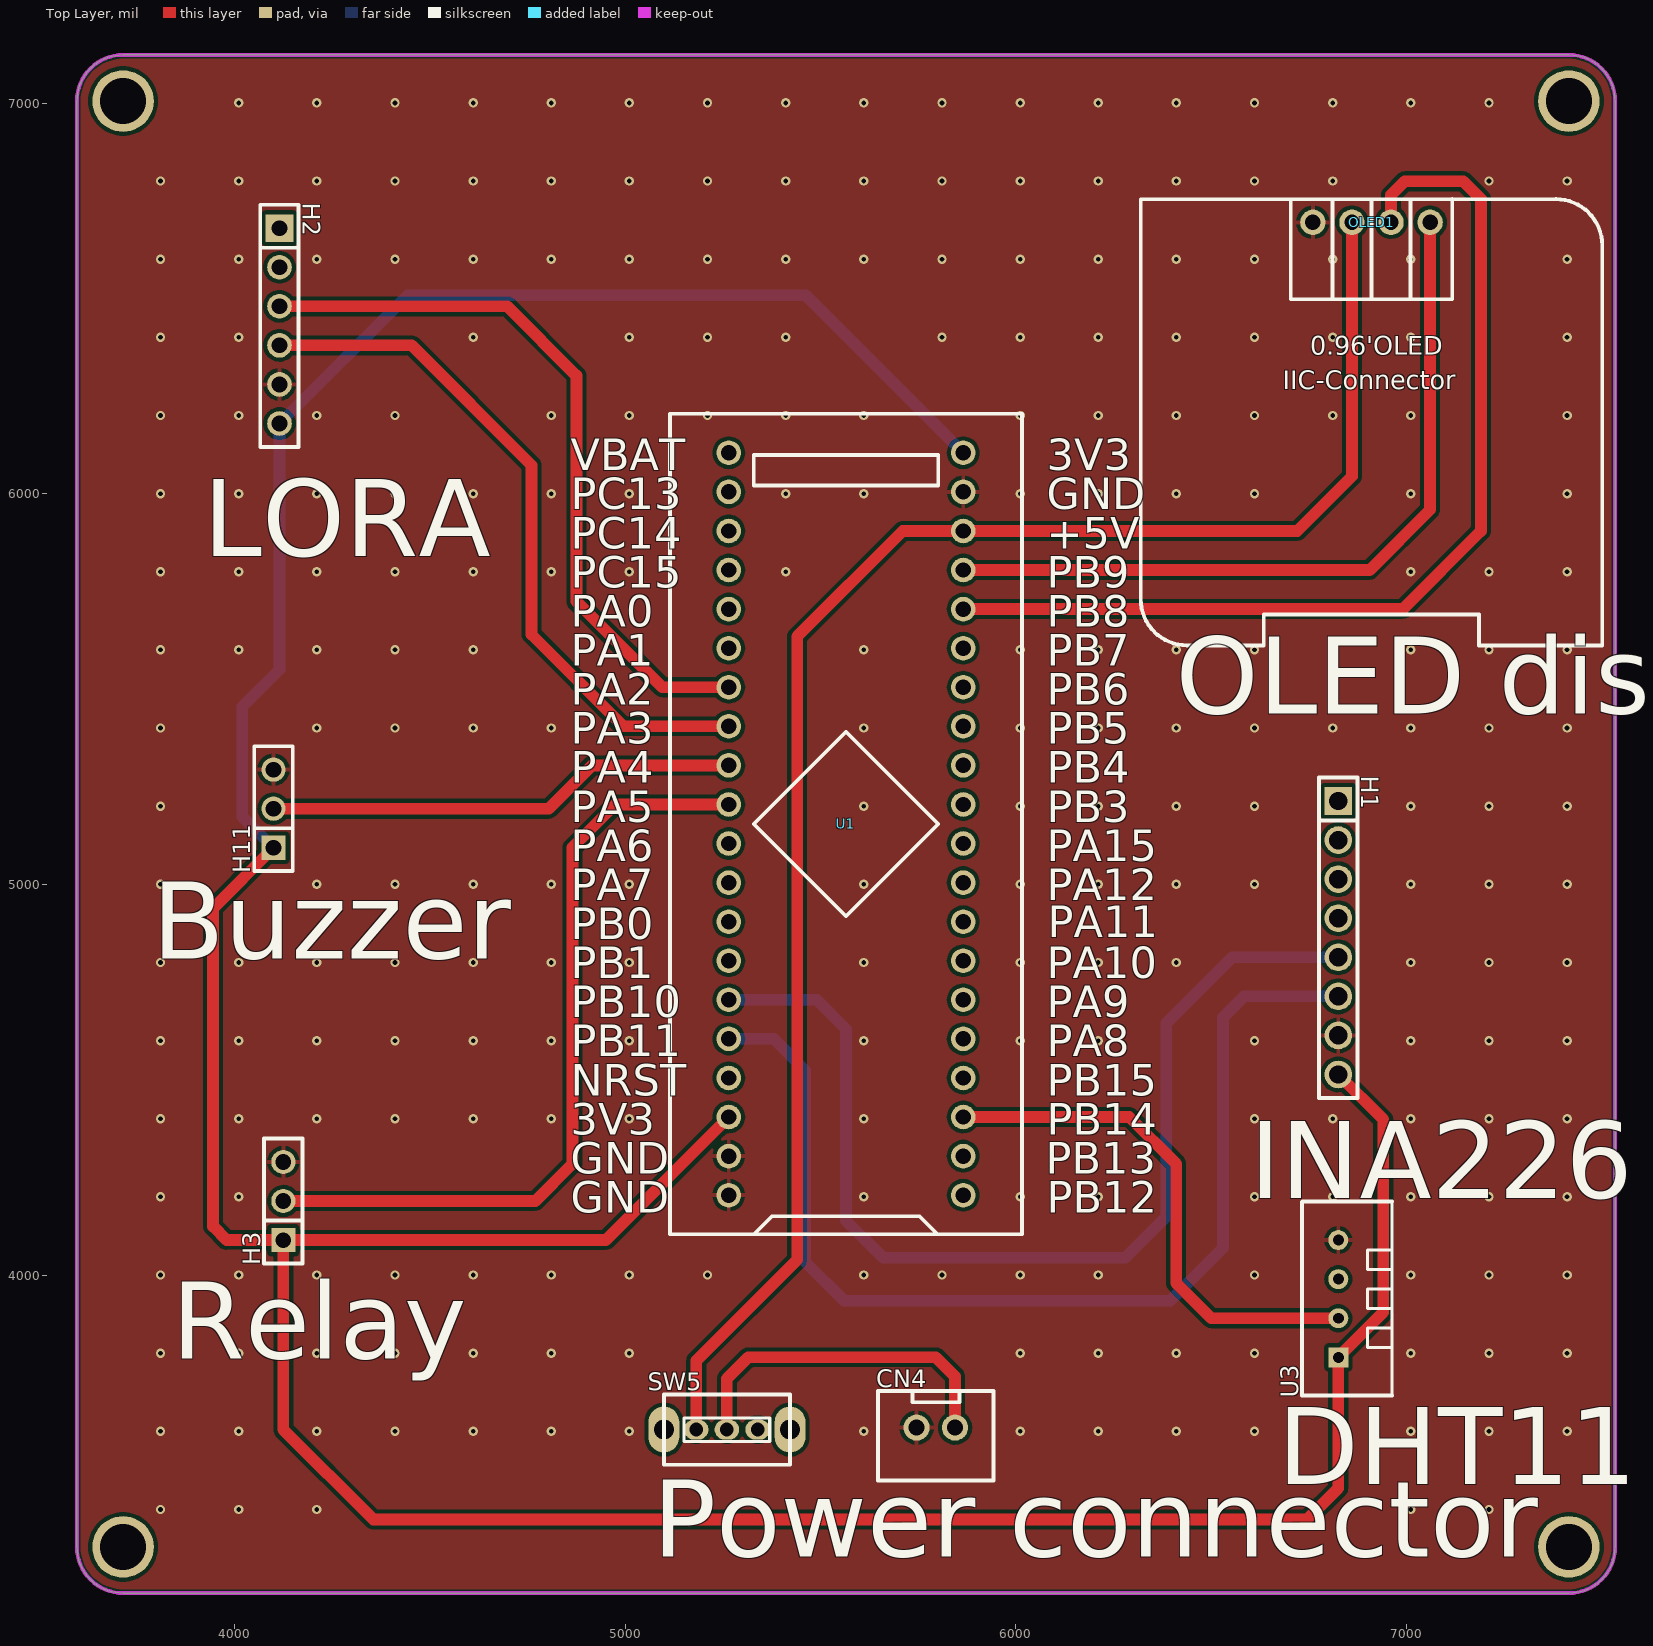
[diagram p0: Top Layer view]
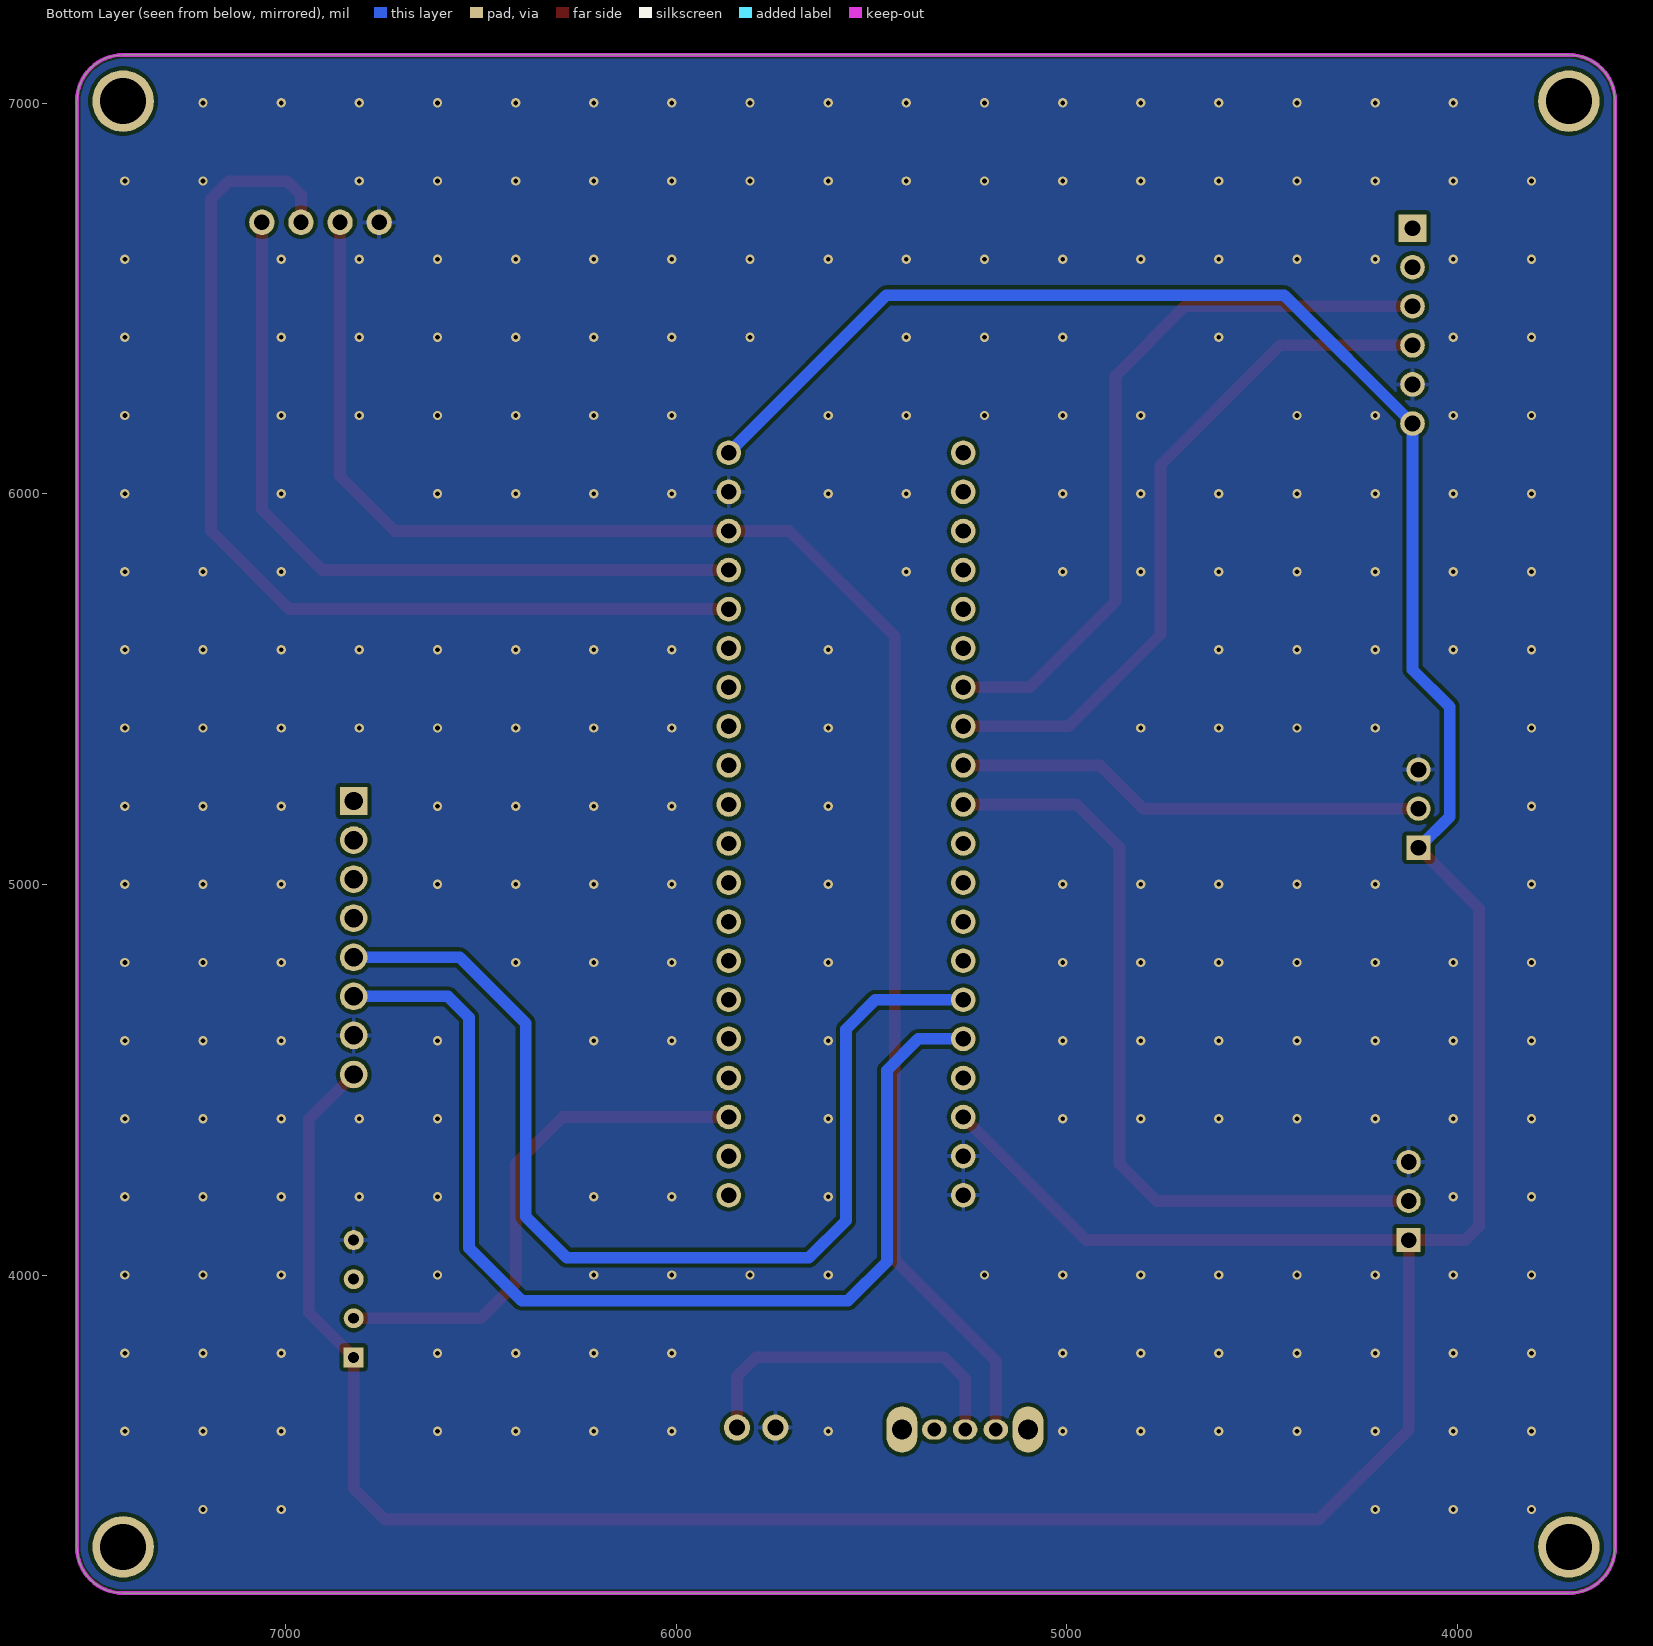
[diagram p1: Bottom Layer view, seen from below]
# Altium PCB MISC51756.pcbdoc
Units mil, origin at the board's own origin, x right, y up, seen from the top; angles counter-clockwise.
Board outline 3937.01 x 3937.01 mil, 2 copper layers (Top Layer, Bottom Layer), stack 62.206 mil thick; 9 components, 38 nets, 79 pads, 261 vias.

## Layer stack, top to bottom
Top Solder Mask Layer: solder mask 0.394, Dk 3.3
Top Layer: signal copper 1.379
Dielectric1: surface 59.449, FR4, Dk 4.5
Bottom Layer: signal copper 1.378
Bottom Solder Mask Layer: solder mask 0.394, Dk 3.3

## Board outline
3714.61,7123.5 ccw(c3714.61,7005.39) 3596.5,7005.39 3596.5,3304.61 ccw(c3714.61,3304.61) 3714.61,3186.5 7415.39,3186.5 ccw(c7415.39,3304.61) 7533.5,3304.61 7533.5,7005.39 ccw(c7415.39,7005.39) 7415.39,7123.5 3714.61,7123.5

## Design rules (kind name [scope] priority, off if disabled: settings)
BoardOutlineClearance copperThickness2oz_1 [All] p2 off: genericclearance=7.99 ignorepadtopadclearanceinfootprint=FALSE except(0: Arc-SplitContinuation Track-SplitContinuation SMDPad-SplitContinuation THPad-SplitContinuation Via-SplitContinuation Fill-SplitContinuation Region-SplitContinuation Poly-SplitContinuation Text-SplitContinuation Hole-SplitContinuation; 5.98: Arc-CutoutEdge Track-CutoutEdge SMDPad-CutoutEdge THPad-CutoutEdge Via-CutoutEdge Text-CutoutEdge; 6.9: Hole-OutlineEdge Hole-CutoutEdge; 10: Poly-OutlineEdge Poly-CutoutEdge; 11.81: Arc-OutlineEdge Track-OutlineEdge SMDPad-OutlineEdge THPad-OutlineEdge Via-OutlineEdge Fill-OutlineEdge Region-OutlineEdge Text-OutlineEdge Fill-CutoutEdge Region-CutoutEdge)
BoardOutlineClearance Plane_innerPlane_1 [All] p4 off: genericclearance=4.02 ignorepadtopadclearanceinfootprint=FALSE except(0: Arc-SplitContinuation Track-SplitContinuation SMDPad-SplitContinuation THPad-SplitContinuation Via-SplitContinuation Fill-SplitContinuation Region-SplitContinuation Poly-SplitContinuation Text-SplitContinuation Hole-SplitContinuation; 5.98: Arc-CutoutEdge Track-CutoutEdge SMDPad-CutoutEdge THPad-CutoutEdge Via-CutoutEdge Text-CutoutEdge; 6.9: Hole-OutlineEdge Hole-CutoutEdge; 10: Poly-OutlineEdge Poly-CutoutEdge; 11.81: Arc-OutlineEdge Track-OutlineEdge SMDPad-OutlineEdge THPad-OutlineEdge Via-OutlineEdge Fill-OutlineEdge Region-OutlineEdge Text-OutlineEdge Fill-CutoutEdge Region-CutoutEdge)
BoardOutlineClearance Copper_copperRegion_1 [All] p6 off: genericclearance=4.02 ignorepadtopadclearanceinfootprint=FALSE except(0: Arc-SplitContinuation Track-SplitContinuation SMDPad-SplitContinuation THPad-SplitContinuation Via-SplitContinuation Fill-SplitContinuation Region-SplitContinuation Poly-SplitContinuation Text-SplitContinuation Hole-SplitContinuation; 5.98: Arc-CutoutEdge Track-CutoutEdge SMDPad-CutoutEdge THPad-CutoutEdge Via-CutoutEdge Text-CutoutEdge; 6.9: Hole-OutlineEdge Hole-CutoutEdge; 10: Poly-OutlineEdge Poly-CutoutEdge; 11.81: Arc-OutlineEdge Track-OutlineEdge SMDPad-OutlineEdge THPad-OutlineEdge Via-OutlineEdge Fill-OutlineEdge Region-OutlineEdge Text-OutlineEdge Fill-CutoutEdge Region-CutoutEdge)
BoardOutlineClearance copperThickness1oz_1 [All] p8: genericclearance=4.02 ignorepadtopadclearanceinfootprint=FALSE except(0: Arc-SplitContinuation Track-SplitContinuation SMDPad-SplitContinuation THPad-SplitContinuation Via-SplitContinuation Fill-SplitContinuation Region-SplitContinuation Poly-SplitContinuation Text-SplitContinuation Hole-SplitContinuation; 5.98: Arc-CutoutEdge Track-CutoutEdge SMDPad-CutoutEdge THPad-CutoutEdge Via-CutoutEdge Text-CutoutEdge; 6.9: Hole-OutlineEdge Hole-CutoutEdge; 10: Poly-OutlineEdge Poly-CutoutEdge; 11.81: Arc-OutlineEdge Track-OutlineEdge SMDPad-OutlineEdge THPad-OutlineEdge Via-OutlineEdge Fill-OutlineEdge Region-OutlineEdge Text-OutlineEdge Fill-CutoutEdge Region-CutoutEdge)
Clearance copperThickness2oz [All] p1 off: gap=7.99 ignorepadtopadclearanceinfootprint=FALSE except(5.98: SMDPad-Track SMDPad-SMDPad THPad-Track SMDPad-THPad THPad-THPad Track-Via SMDPad-Via THPad-Via Via-Via Fill-SMDPad Region-SMDPad Fill-THPad Region-THPad Fill-Via Region-Via Fill-Fill Fill-Region Region-Region Arc-Track Arc-SMDPad Arc-THPad Arc-Via Fill-Arc Region-Arc Arc-Arc Text-Track SMDPad-Text Text-THPad Text-Via Fill-Text Region-Text Arc-Text Text-Text; 6.9: Hole-Track Hole-SMDPad Hole-THPad Hole-Via Fill-Hole Region-Hole Hole-Arc Hole-Text; 10: Poly-Track Poly-SMDPad Poly-THPad Poly-Via Poly-Fill Poly-Region Poly-Poly Poly-Arc Poly-Text Poly-Hole; 11.81: Fill-Track Region-Track)
Clearance Plane_innerPlane [All] p3 off: gap=4.02 ignorepadtopadclearanceinfootprint=FALSE except(5.98: SMDPad-Track SMDPad-SMDPad THPad-Track SMDPad-THPad THPad-THPad Track-Via SMDPad-Via THPad-Via Via-Via Fill-SMDPad Region-SMDPad Fill-THPad Region-THPad Fill-Via Region-Via Fill-Fill Fill-Region Region-Region Arc-Track Arc-SMDPad Arc-THPad Arc-Via Fill-Arc Region-Arc Arc-Arc Text-Track SMDPad-Text Text-THPad Text-Via Fill-Text Region-Text Arc-Text Text-Text; 6.9: Hole-Track Hole-SMDPad Hole-THPad Hole-Via Fill-Hole Region-Hole Hole-Arc Hole-Text; 10: Poly-Track Poly-SMDPad Poly-THPad Poly-Via Poly-Fill Poly-Region Poly-Poly Poly-Arc Poly-Text Poly-Hole; 11.81: Fill-Track Region-Track)
Clearance Copper_copperRegion [All] p5 off: gap=4.02 ignorepadtopadclearanceinfootprint=FALSE except(5.98: SMDPad-Track SMDPad-SMDPad THPad-Track SMDPad-THPad THPad-THPad Track-Via SMDPad-Via THPad-Via Via-Via Fill-SMDPad Region-SMDPad Fill-THPad Region-THPad Fill-Via Region-Via Fill-Fill Fill-Region Region-Region Arc-Track Arc-SMDPad Arc-THPad Arc-Via Fill-Arc Region-Arc Arc-Arc Text-Track SMDPad-Text Text-THPad Text-Via Fill-Text Region-Text Arc-Text Text-Text; 6.9: Hole-Track Hole-SMDPad Hole-THPad Hole-Via Fill-Hole Region-Hole Hole-Arc Hole-Text; 10: Poly-Track Poly-SMDPad Poly-THPad Poly-Via Poly-Fill Poly-Region Poly-Poly Poly-Arc Poly-Text Poly-Hole; 11.81: Fill-Track Region-Track)
Clearance copperThickness1oz [All] p7: gap=4.02 ignorepadtopadclearanceinfootprint=FALSE except(5.98: SMDPad-Track SMDPad-SMDPad THPad-Track SMDPad-THPad THPad-THPad Track-Via SMDPad-Via THPad-Via Via-Via Fill-SMDPad Region-SMDPad Fill-THPad Region-THPad Fill-Via Region-Via Fill-Fill Fill-Region Region-Region Arc-Track Arc-SMDPad Arc-THPad Arc-Via Fill-Arc Region-Arc Arc-Arc Text-Track SMDPad-Text Text-THPad Text-Via Fill-Text Region-Text Arc-Text Text-Text; 6.9: Hole-Track Hole-SMDPad Hole-THPad Hole-Via Fill-Hole Region-Hole Hole-Arc Hole-Text; 10: Poly-Track Poly-SMDPad Poly-THPad Poly-Via Poly-Fill Poly-Region Poly-Poly Poly-Arc Poly-Text Poly-Hole; 11.81: Fill-Track Region-Track)
DiffPairsRouting differentialPair [All] p1: maxlimit=6 minlimit=6 mostfreqgap=6 toplayer_minwidth=5 toplayer_prefwidth=10 toplayer_maxwidth=100 toplayer_mingap=6 toplayer_prefgap=6 toplayer_maxgap=6 bottomlayer_minwidth=5 bottomlayer_prefwidth=10 bottomlayer_maxwidth=100 bottomlayer_mingap=6 bottomlayer_prefgap=6 bottomlayer_maxgap=6 maxuncoupledlength=10
HoleToHoleClearance otherClearance [All] p1: gap=11.81 allowstackedmicrovias=TRUE
Length netLength [All] p1: minlimit=0 maxlimit=0
PasteMaskExpansion pasteMaskExpansion [All] p1: expansion=0
PlaneConnect innerPlane [All] p1: planeconnectstyle=Relief reliefexpansion=20 reliefentries=4 reliefconductorwidth=10 reliefairgap=10
PolygonConnect copperRegion [All] p1: connectstyle=Relief reliefconductorwidth=10 reliefentries=4 polygonreliefangle="90 Angle" airgapwidth=10 via.connectstyle=Relief via.reliefconductorwidth=10 via.reliefentries=4 via.polygonreliefangle="90 Angle" via.airgapwidth=10
RoutingVias viaSize [All] p1: holewidth=12.01 width=24.02 viastyle="Through Hole" minholewidth=11.81 minwidth=19.68 maxholewidth=248.03 maxwidth=393.7
SolderMaskExpansion solderMaskExpansion [IsVia] p1: expansion=-1000 istentingtop=TRUE
SolderMaskExpansion solderMaskExpansion [All] p2: expansion=2 istentingtop=FALSE
Width copperThickness2oz_2 [All] p1 off: maxlimit=100 minlimit=8 preferedwidth=10
Width copperThickness1oz_2 [All] p2: maxlimit=100 minlimit=5 preferedwidth=10

## Components (designator, comment, footprint, x,y, rotation, side; value= is the part's Value field where it differs from the comment)
CN4 "XH2.54*2P_Through-hole" CONN-TH_2P-P2.50-XH2.54-2P 5795,3610 r0 top
H1 "" HDR-TH_8P-P2.54-V-F-1 6825,4863.84 r270 top
H2 "" HDR-TH_6P-P2.54-V-F 4115,6430 r270 top
H3 "" HDR-TH_3P-P2.54-V-F 4125,4190 r90 top
H11 "" HDR-TH_3P-P2.54-V-F 4099.74,5194.14 r90 top
OLED1 "" 0.96OLED_4P 6910,6695 r0 top
SW5 "" 拨动开关 5255,3605 r0 top
U1 "STM32F103C8T6-Card" CONN-TH_L53.3-W22.9_STM32F103C8T6-CARD 5565,5155 r90 top
U3 "DHT11" SENSOR-TH_DHT11 6825,3940 r90 top

## Footprints (in the part's own frame and the unit in brackets; to place one, negate y for a bottom-side part, rotate by r counter-clockwise, add the part's x,y. Pads: shape width x height; smd on the part's side, far side on the other; paste and mask are expansions set on the pad)
0.96OLED_4P [mm]
  round 1.65 hole 1 copper offset 0,0: 1(-3.81,-0.001) 2(-1.27,0.002) 3(1.27,0.002) 4(3.81,0.002)
  silkscreen extent -15,-27.5 15,1.5
CONN-TH_2P-P2.50-XH2.54-2P [mm]
  round 1.7 hole 1.05 paste+0 mask+0.05: 1(1.25,0) 2(-1.25,0)
  silkscreen extent -3.75,-3.42 3.75,2.37
CONN-TH_L53.3-W22.9_STM32F103C8T6-CARD [mm]
  round 1.6 hole 1: 1(-24.13,-7.62) 2(-21.59,-7.62) 3(-19.05,-7.62) 4(-16.51,-7.62) 5(-13.97,-7.62) 6(-11.43,-7.62) 7(-8.89,-7.62) 8(-6.35,-7.62) 9(-3.81,-7.62) 10(-1.27,-7.62) 11(1.27,-7.62) 12(3.81,-7.62) 13(6.35,-7.62) 14(8.89,-7.62) 15(11.43,-7.62) 16(13.97,-7.62) 17(16.51,-7.62) 18(19.05,-7.62) 19(21.59,-7.62) 20(24.13,-7.62) 21(24.13,7.62) 22(21.59,7.62) 23(19.05,7.62) 24(16.51,7.62) 25(13.97,7.62) 26(11.43,7.62) 27(8.89,7.62) 28(6.35,7.62) 29(3.81,7.62) 30(1.27,7.62) 31(-1.27,7.62) 32(-3.81,7.62) 33(-6.35,7.62) 34(-8.89,7.62) 35(-11.43,7.62) 36(-13.97,7.62) 37(-16.51,7.62) 38(-19.05,7.62) 39(-21.59,7.62) 40(-24.13,7.62)
  silkscreen extent -26.67,-11.43 26.67,11.43
HDR-TH_3P-P2.54-V-F [mil]
  rect 62x62 hole 40.16: 1(-100,0)
  round 62 hole 40.16: 2(0,0) 3(100,0)
  silkscreen extent -160,-49 160,49
HDR-TH_6P-P2.54-V-F [mm]
  rect 1.8x1.8 hole 1.02: 1(-6.35,0)
  round 1.6 hole 1.02: 2(-3.81,0) 3(-1.27,0) 4(1.27,0) 5(3.81,0) 6(6.35,0)
  silkscreen extent -7.87,-1.25 7.87,1.25
HDR-TH_8P-P2.54-V-F-1 [mm]
  rect 1.8x1.8 hole 1.2: 1(-8.89,0)
  round 1.8 hole 1.2: 2(-6.35,0) 3(-3.81,0) 4(-1.27,0) 5(1.27,0) 6(3.81,0) 7(6.35,0) 8(8.89,0)
  silkscreen extent -10.41,-1.25 10.41,1.25
SENSOR-TH_DHT11 [mil]
  rect 51x51 hole 28: 1(-150,0)
  round 51 hole 28: 2(-50,0) 3(50,0) 4(150,0)
  silkscreen extent -248,-138 248,93
拨动开关 [mil]
  oval 63x51.2 hole 35.4 paste+0 mask+2: 1(-73.4,0) 2(5,0) 3(84,0)
  oval 78.7x118.1 hole 51.2 paste+0 mask+2: 4(166.7,0) 5(-156.1,0)
  silkscreen extent -156,-90 167,90

## Free pads (board coordinates)
  round 157.48 hole 118.11: 1(3714.61,7005.39) 1(3714.61,3304.61) 1(7415.39,7005.39) 1(7415.39,3304.61)

## Via types
v1: diameter 24.02, hole 12, Top Layer to Bottom Layer, 261 vias

## Nets (pads, with @x,y where several pads share a name; then routed paths per layer and width w, separated by ;. In a path a pad name is that pad's centre, name@x,y a point inside that pad or via, vN(x,y) a via of type N, cw(c..) or ccw(c..) an arc to the next point about the centre after c; other vN are vias at no path point)
$1N17136: CN4.1 SW5.2 | length 888.2
  Top Layer w30: SW5.2 5260,3735 5315,3790 5795,3790 5844.22,3740.78 CN4.1
+5V: OLED1.2 SW5.1 U1.18 | length 4376.9
  Top Layer w30: SW5.1 5181.6,3781.6 5440,4040 5440,5635 5710,5905 U1.18 6720,5905 6860,6045 OLED1.2@6860,6695.05
GND: CN4.2 H1.7 H2.5 H3.3 H11.3 OLED1.1 U1.19 U1.39 U1.40 U3.4
  other v1: 3810.6,3400.6 4010.6,3400.6 4210.6,3400.6 7010.6,3400.6 7210.6,3400.6 3810.6,3600.6 4010.6,3600.6 4210.6,3600.6 4410.6,3600.6 4610.6,3600.6 4810.6,3600.6 5010.6,3600.6 5610.6,3600.6 6010.6,3600.6 6210.6,3600.6 6410.6,3600.6 6610.6,3600.6 7010.6,3600.6 7210.6,3600.6 7410.6,3600.6 3810.6,3800.6 4010.6,3800.6 4210.6,3800.6 4410.6,3800.6 4610.6,3800.6 4810.6,3800.6 5010.6,3800.6 6010.6,3800.6 6210.6,3800.6 6410.6,3800.6 6610.6,3800.6 7010.6,3800.6 7210.6,3800.6 7410.6,3800.6 3810.6,4000.6 4010.6,4000.6 4210.6,4000.6 4410.6,4000.6 4610.6,4000.6 4810.6,4000.6 5010.6,4000.6 5210.6,4000.6 5610.6,4000.6 5810.6,4000.6 6010.6,4000.6 6210.6,4000.6 6610.6,4000.6 7010.6,4000.6 7210.6,4000.6 7410.6,4000.6 3810.6,4200.6 4010.6,4200.6 5610.6,4200.6 6010.6,4200.6 6210.6,4200.6 6610.6,4200.6 6810.6,4200.6 7010.6,4200.6 7210.6,4200.6 7410.6,4200.6 3810.6,4400.6 4010.6,4400.6 4210.6,4400.6 4410.6,4400.6 4610.6,4400.6 4810.6,4400.6 5010.6,4400.6 5610.6,4400.6 6610.6,4400.6 6810.6,4400.6 7010.6,4400.6 7210.6,4400.6 7410.6,4400.6 3810.6,4600.6 4010.6,4600.6 4210.6,4600.6 4410.6,4600.6 4610.6,4600.6 4810.6,4600.6 5010.6,4600.6 5610.6,4600.6 6010.6,4600.6 6210.6,4600.6 6610.6,4600.6 7010.6,4600.6 7210.6,4600.6 7410.6,4600.6 3810.6,4800.6 4010.6,4800.6 4210.6,4800.6 4410.6,4800.6 4610.6,4800.6 4810.6,4800.6 5010.6,4800.6 5610.6,4800.6 6010.6,4800.6 6210.6,4800.6 6410.6,4800.6 7010.6,4800.6 7210.6,4800.6 7410.6,4800.6 3810.6,5000.6 4210.6,5000.6 4410.6,5000.6 4610.6,5000.6 4810.6,5000.6 5010.6,5000.6 5610.6,5000.6 6010.6,5000.6 6210.6,5000.6 6410.6,5000.6 6610.6,5000.6 7010.6,5000.6 7210.6,5000.6 7410.6,5000.6 3810.6,5200.6 5610.6,5200.6 6010.6,5200.6 6210.6,5200.6 6410.6,5200.6 6610.6,5200.6 7010.6,5200.6 7210.6,5200.6 7410.6,5200.6 3810.6,5400.6 4210.6,5400.6 4410.6,5400.6 4610.6,5400.6 4810.6,5400.6 5610.6,5400.6 6010.6,5400.6 6210.6,5400.6 6410.6,5400.6 6610.6,5400.6 6810.6,5400.6 7010.6,5400.6 7210.6,5400.6 7410.6,5400.6 3810.6,5600.6 4010.6,5600.6 4210.6,5600.6 4410.6,5600.6 4610.6,5600.6 5610.6,5600.6 6010.6,5600.6 6210.6,5600.6 6410.6,5600.6 6610.6,5600.6 6810.6,5600.6 7010.6,5600.6 7210.6,5600.6 7410.6,5600.6 3810.6,5800.6 4010.6,5800.6 4210.6,5800.6 4410.6,5800.6 4610.6,5800.6 4810.6,5800.6 5010.6,5800.6 5410.6,5800.6 7010.6,5800.6 7210.6,5800.6 7410.6,5800.6 3810.6,6000.6 4010.6,6000.6 4210.6,6000.6 4410.6,6000.6 4610.6,6000.6 4810.6,6000.6 5010.6,6000.6 5410.6,6000.6 5610.6,6000.6 6010.6,6000.6 6210.6,6000.6 6410.6,6000.6 6610.6,6000.6 7010.6,6000.6 7410.6,6000.6 3810.6,6200.6 4010.6,6200.6 4210.6,6200.6 4410.6,6200.6 4810.6,6200.6 5010.6,6200.6 5210.6,6200.6 5410.6,6200.6 5610.6,6200.6 6010.6,6200.6 6210.6,6200.6 6410.6,6200.6 6610.6,6200.6 6810.6,6200.6 7010.6,6200.6 7410.6,6200.6 3810.6,6400.6 4010.6,6400.6 4610.6,6400.6 5010.6,6400.6 5210.6,6400.6 5410.6,6400.6 5810.6,6400.6 6010.6,6400.6 6210.6,6400.6 6410.6,6400.6 6610.6,6400.6 6810.6,6400.6 7010.6,6400.6 7410.6,6400.6 3810.6,6600.6 4010.6,6600.6 4210.6,6600.6 4410.6,6600.6 4610.6,6600.6 4810.6,6600.6 5010.6,6600.6 5210.6,6600.6 5410.6,6600.6 5610.6,6600.6 5810.6,6600.6 6010.6,6600.6 6210.6,6600.6 6410.6,6600.6 6610.6,6600.6 6810.6,6600.6 7010.6,6600.6 7410.6,6600.6 3810.6,6800.6 4010.6,6800.6 4210.6,6800.6 4410.6,6800.6 4610.6,6800.6 4810.6,6800.6 5010.6,6800.6 5210.6,6800.6 5410.6,6800.6 5610.6,6800.6 5810.6,6800.6 6010.6,6800.6 6210.6,6800.6 6410.6,6800.6 6610.6,6800.6 6810.6,6800.6 7210.6,6800.6 7410.6,6800.6 4010.6,7000.6 4210.6,7000.6 4410.6,7000.6 4610.6,7000.6 4810.6,7000.6 5010.6,7000.6 5210.6,7000.6 5410.6,7000.6 5610.6,7000.6 5810.6,7000.6 6010.6,7000.6 6210.6,7000.6 6410.6,7000.6 6610.6,7000.6 6810.6,7000.6 7010.6,7000.6 7210.6,7000.6
NRST: U1.37
PA0: U1.25
PA1: U1.26
PA2: H2.3 U1.27 | length 1892.3
  Top Layer w30: H2.3 4697.7,6480 4875,6302.7 4875,5725 5095,5505 U1.27
PA3: H2.4 U1.28 | length 1807.6
  Top Layer w30: H2.4 4453.21,6380 4760,6073.21 4760,5640 4995,5405 U1.28
PA4: H11.2 U1.29 | length 1211.2
  Top Layer w30: H11.2 4804.14,5194.14 4915,5305 U1.29
PA5: H3.2 U1.30 | length 2034.9
  Top Layer w30: H3.2 4770,4190 4865,4285 4865,5095 4975,5205 U1.30
PA6: U1.31
PA7: U1.32
PA8: U1.5
PA9: U1.6
PA10: U1.7
PA11: U1.8
PA12: U1.9
PA15: U1.10
PB0: U1.33
PB1: U1.34
PB3: U1.11
PB4: U1.12
PB5: U1.13
PB6: U1.14
PB7: U1.15
PB8: OLED1.3 U1.16 | length 2590.9
  Top Layer w30: U1.16 6990,5705 7190,5905 7190,6755 7145,6800 6995,6800 6960,6765 OLED1.3@6960,6695.05
PB9: OLED1.4 U1.17 | length 1994.3
  Top Layer w30: U1.17 6905,5805 7060,5960 OLED1.4@7060,6695.05
PB10: H1.5 U1.35 | length 2728.8
  Bottom Layer w30: U1.35 5490,4705 5565,4630 5565,4140 5660,4045 6280,4045 6385,4150 6385,4645 6553.84,4813.84 H1.5
PB11: H1.6 U1.36 | length 2792.8
  Bottom Layer w30: U1.36 5380,4605 5460,4525 5460,4035 5560,3935 6395,3935 6530,4070 6530,4660 6583.84,4713.84 H1.6
PB12: U1.1
PB13: U1.2
PB14: U1.3 U3.2 | length 1352
  Top Layer w30: U1.3 6290,4405 6410,4285 6410,3980 6500,3890 U3.2
PB15: U1.4
PC13: U1.22
PC14: U1.23
PC15: U1.24
VBAT: U1.21
VCC: H1.8 H2.6 H3.1 H11.1 U1.20 U1.38 U3.1 | length 10176.9
  Top Layer w30: H11.1 3945,4939.4 3945,4125 3980,4090 H3.1 ; U1.38 4950,4090 H3.1 ; H1.8 6940,4398.84 6940,3905 U3.1 6825,3455 6745,3375 4355,3375 4125,3605 H3.1
  Bottom Layer w30: H11.1 4020,5173.88 4020,5455 4115,5550 H2.6 4443.21,6508.21 5461.79,6508.21 U1.20
pads on no net: H1.1 H1.2 H1.3 H1.4 H2.1 H2.2 SW5.3 SW5.4 SW5.5 U3.3

## Polygon pours and split planes (outlines as drawn)
GND on Bottom Layer (solid, remove dead copper, pour order 2): 3525,7245 3525,3080 7700,3080 7700,7245
GND on Top Layer (solid, remove dead copper, pour order 2): 3000,7415 3000,3000 7930,3000 7930,7415

## Keep-outs
Board Outline Layer:
  the board outline again, w10

## Silkscreen, mask and mechanical layers (free items; w line width, h text height)
Top Silkscreen Layer:
  text "VBAT" at 4860.95,6060 h80
  text "3V3" at 6079.16,6060 h80
  text "PC13" at 4860.95,5960 h80
  text "GND" at 6079.16,5960 h80
  text "PC14" at 4860.95,5860 h80
  text "+5V" at 6079.16,5860 h80
  text "LORA" at 3920,5840 h196.85
  text "PC15" at 4860.95,5760 h80
  text "PB9" at 6079.16,5760 h80
  text "PA0" at 4860.95,5660 h80
  text "PB8" at 6079.16,5660 h80
  text "PA1" at 4860.95,5560 h80
  text "PB7" at 6079.16,5560 h80
  text "PA2" at 4860.95,5460 h80
  text "PB6" at 6079.16,5460 h80
  text "OLED display" at 6408.66,5436.57 h196.85
  text "PA3" at 4860.95,5360 h80
  text "PB5" at 6079.16,5360 h80
  text "PA4" at 4860.95,5260 h80
  text "PB4" at 6079.16,5260 h80
  text "PA5" at 4860.95,5160 h80
  text "PB3" at 6079.16,5160 h80
  text "PA6" at 4860.95,5060 h80
  text "PA15" at 6079.16,5060 h80
  text "PA7" at 4860.95,4960 h80
  text "PA12" at 6079.16,4960 h80
  text "PA11" at 6080.95,4865 h80
  text "PB0" at 4860.95,4860 h80
  text "Buzzer" at 3790,4810 h196.85
  text "PB1" at 4860.95,4760 h80
  text "PA10" at 6079.16,4760 h80
  text "PB10" at 4860.95,4660 h80
  text "PA9" at 6079.16,4660 h80
  text "PB11" at 4860.95,4560 h80
  text "PA8" at 6079.16,4560 h80
  text "NRST" at 4860.95,4460 h80
  text "PB15" at 6079.16,4460 h80
  text "3V3" at 4860.95,4360 h80
  text "PB14" at 6079.16,4360 h80
  text "GND" at 4860.95,4260 h80
  text "PB13" at 6075.95,4260 h80
  text "INA226" at 6598.94,4196.57 h196.85
  text "GND" at 4860.95,4160 h80
  text "PB12" at 6079.16,4160 h80
  text "Relay" at 3839.72,3786.57 h196.85
  text "DHT11" at 6670,3465 h196.85
  text "Power connector" at 5070,3280 h196.85